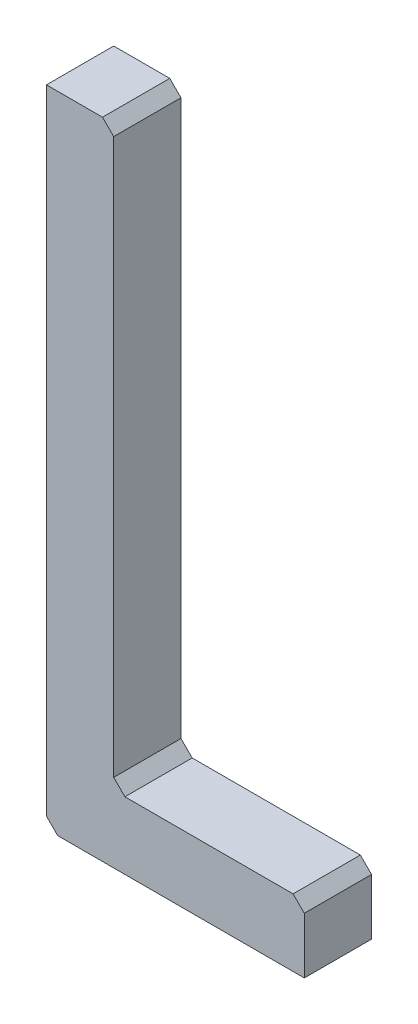
from build123d import *

# Parameters (mm, degrees)
EXTRUDE_1_DEPTH = 6
CHAMFER_1_SIZE  = 2
CHAMFER_2_SIZE  = 2
CHAMFER_3_SIZE  = 2


with BuildPart() as part:
    # 草图1 → 凸台-拉伸1 (new, symmetric)
    with BuildSketch(Plane.XY):
        Polygon((0, 0), (0, 115), (12, 115), (12, 12), (46, 12), (46, 0), align=None)
    extrude(amount=EXTRUDE_1_DEPTH, both=True)

    # 倒角1
    chamfer_1_edges = [part.edges().sort_by_distance(p)[0] for p in [
        (12, 12, 0),
    ]]
    chamfer(chamfer_1_edges, length=CHAMFER_1_SIZE)

    # 倒角2
    chamfer_2_edges = [part.edges().sort_by_distance(p)[0] for p in [
        (0, 0, 0),
    ]]
    chamfer(chamfer_2_edges, length=CHAMFER_2_SIZE)

    # 倒角3
    chamfer_3_edges = [part.edges().sort_by_distance(p)[0] for p in [
        (12, 115, 0),
        (46, 12, 0),
    ]]
    chamfer(chamfer_3_edges, length=CHAMFER_3_SIZE)


solid = part.part
